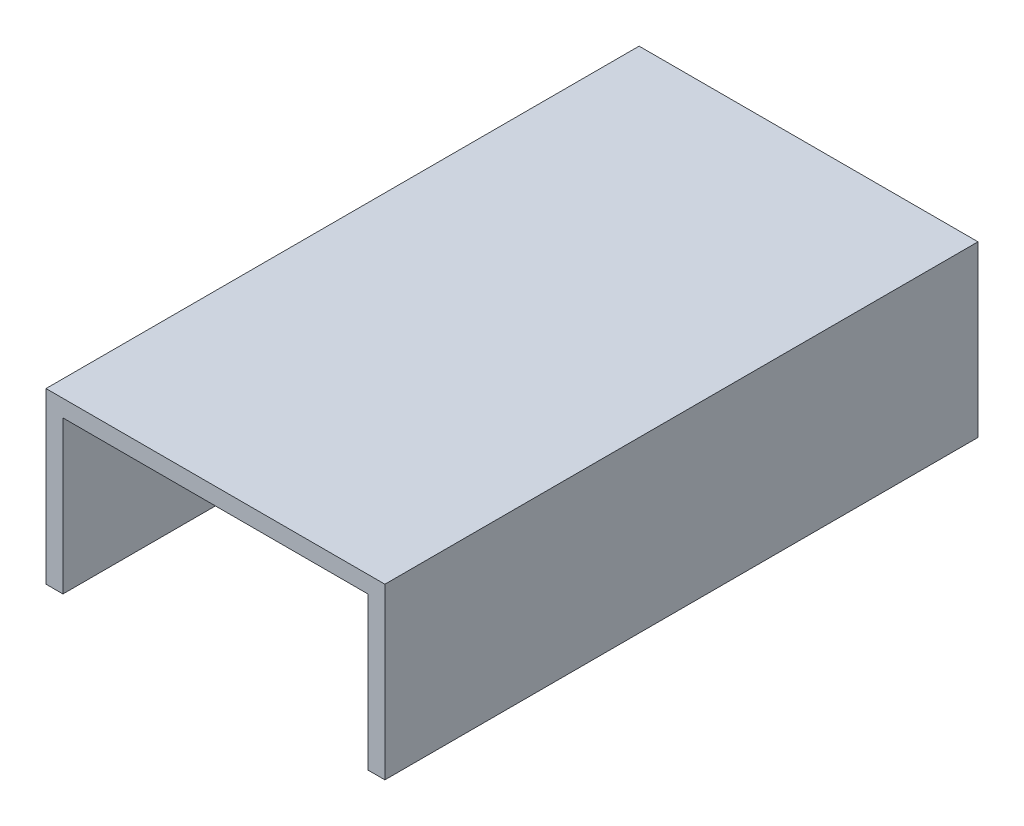
SolidWorks part; units mm, degrees
ref_plane "前视基准面" through (0, 0, 0) normal (0, 0, 1) x (1, 0, 0)
ref_plane "上视基准面" through (0, 0, 0) normal (0, 1, 0) x (1, 0, 0)
ref_plane "右视基准面" through (0, 0, 0) normal (1, 0, 0) x (0, 0, -1)
sketch "草图1" plane through (0, 0, 0) normal (0, 0, 1) x (1, 0, 0)
  line L0 (0, 0) -> (100, 0)
  line L1 (100, 0) -> (100, -50)
  line L2 (0, 0) -> (0, -50)
  line L3 (5, -5) -> (5, -50)
  line L4 (5, -5) -> (95, -5)
  line L5 (95, -5) -> (95, -50)
  line L6 (0, -50) -> (5, -50)
  line L7 (95, -50) -> (100, -50)
  dimension "D1" = 5
extrude "凸台-拉伸1" add sketch "草图1" along normal blind 175
